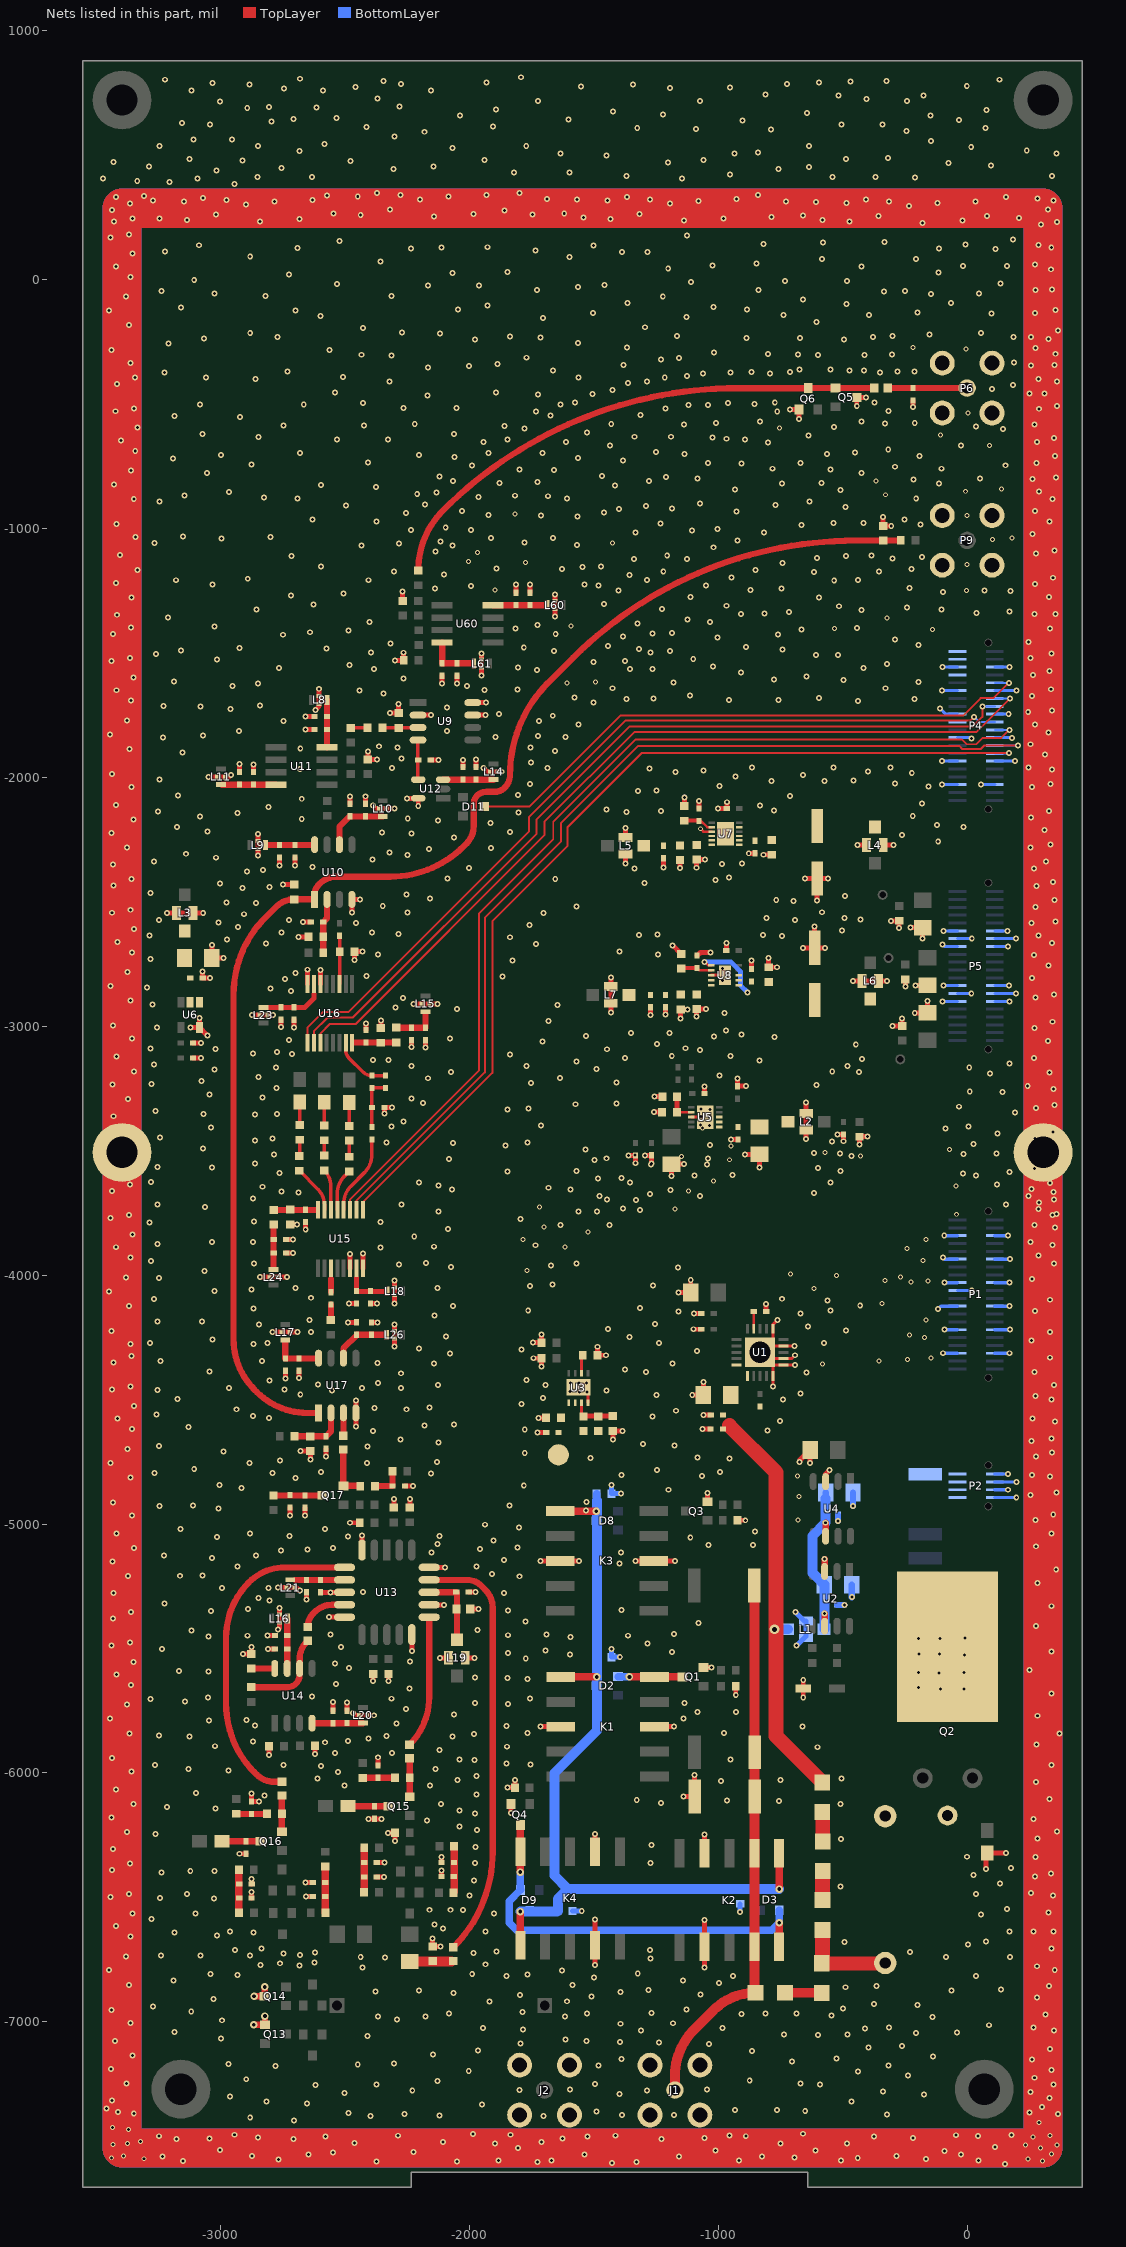
[diagram p0: the nets of this part, all layers, seen from the top]
# Altium PCB MISC109358.PcbDoc (part 5 of 7)
Units mil, origin at the board's own origin, x right, y up, seen from the top; angles counter-clockwise.
Board outline 4015.75 x 8543.31 mil, 4 copper layers (TopLayer, GND, POWER, BottomLayer), stack 33.234 mil thick; 299 components, 170 nets, 998 pads, 2318 vias.

## Via types
v1: diameter 24, hole 12, TopLayer to BottomLayer, 2184 vias
v2: diameter 20, hole 12, TopLayer to BottomLayer, 95 vias
v3: diameter 30, hole 15, TopLayer to BottomLayer, 37 vias
v4: diameter 40, hole 20, TopLayer to BottomLayer, 2 vias

## Nets (pads, with @x,y where several pads share a name; then routed paths per layer and width w, separated by ;. In a path a pad name is that pad's centre, name@x,y a point inside that pad or via, vN(x,y) a via of type N, cw(c..) or ccw(c..) an arc to the next point about the centre after c; other vN are vias at no path point) (continued)
GND: (continued)
  other v1: -2432.52,-301.52 -679,-301 -301,-301 -800,-299 355.48,-297.52 -1018,-292 -3438.52,-282.52 -2562.52,-282.52 275.48,-273.52 -1367.52,-271.52 -3208.52,-255.52 -1563.52,-254.52 -495.52,-240.52 -1977.52,-239.52 327.48,-238.52 -3066.52,-236.52 -887,-234 -671.52,-233.52 -1715,-232 -2770.52,-230.52 -379,-230 185.48,-230.52 257.48,-229.52 -1836.52,-227.52 -1165,-227 -299.52,-225.52 -150.52,-220.52 -2117.52,-216.52 -2880.52,-214.52 56.48,-214.52 -2270.52,-211.52 365.48,-204.52 -2426.85,-193.52 -1295,-191 -3368.52,-182.52 -606,-169 -1704.52,-154.52 -1127,-150 -2597.52,-145.52 -738,-142 -395,-142 97,-136 -1503,-134 272,-134 -199,-132 -3447.52,-123.52 -2699.52,-123.52 355,-122 -2045.52,-120.52 -884,-119 -3159.3,-111.52 -1020,-109 -1926.52,-103.52 -485,-97 -1365,-93 -64,-93 -660,-80 -1223,-68 -3379.52,-67.52 -2819.52,-65.52 -2313.52,-65.52 -146,-57 47,-55 -3023.52,-54.52 -335,-47 -3236.52,-45.52 -249,-45 274,-42 -839,-41 -1728.52,-40.52 341,-39 -1563,-29 -2165.52,-23.52 -1961.52,-23.52 -1458,-21 -2532.16,-17.52 134,-16 -1110,-10 -732,-6 -483,-6 -3105.52,-1.52 -3362.52,11.48 -2724.52,21.48 -2068.52,27.48 -115,29 -1847.31,30.48 337,42 -1201,45 -425,53 -3420.52,53.48 -16,56 161,56 -1024,58 273,62 -847,66 -2356.52,73.48 -584,84 -205,84 -1598,91 -2880.52,92.48 -3353.52,104.48 -1386,111 -1285,111 -3222.52,113.48 -1734.52,116.48 113,123 -2234,124.48 -113,125 -2691.52,127.48 -2111.52,129.48 338,130 -1927.52,130.48 -1501,138 -3085.52,138.48 286,140 -6,142 -818,144 -580,150 -333,152 -2522.52,155.48 185,162 -3441.52,170.48 -1125,177 -3367.52,182.48 297.48,221.48 -178.52,228.48 360.48,231.48 -3427.52,233.48 -2841.52,234.48 -472.52,234.48 -1138.52,237.48 -19.52,237.48 -3135.52,240.48 -581.52,240.48 -2682.52,243.48 -1432.52,243.48 -3354.52,245.48 -3244.52,246.48 -979.52,246.48 208.48,247.48 -1541.52,249.48 -785.52,252.48 -2142.52,254.48 -355.52,255.48 79.48,255.48 -658.83,257.48 -2436.52,260.48 -3018.52,261.48 -1745.52,261.48 -1983.52,263.48 -1315.52,264.48 -2545.52,266.48 -1618.83,266.48 -1858.52,278.48 -3435.52,279.48 -2319.52,281.48 324.48,281.48 -234.52,296.48 -2897.52,302.48 -3363.52,305.48 -1194.52,305.48 -119.52,307.48 -484.52,308.48 -607.52,312.48 -2782.52,313.48 -313.52,313.48 -3147.52,314.48 -727.52,314.48 33.48,314.48 -1079.52,316.48 -1444.52,317.48 -3270.52,318.48 346.48,318.48 -2976.52,319.48 -2629.52,320.48 -1567.52,321.48 -2198.52,322.48 -1273.52,322.48 -406.52,322.48 -1687.52,323.48 -926.52,323.48 282.03,325.48 -3069.52,328.48 -3419.52,331.48 -1366.52,331.48 155.48,332.48 -2083.52,333.48 -2448.52,334.48 -3308.19,336.48 -2571.52,338.48 -2277.52,339.48 -839.52,339.48 -1930.52,340.48 -2370.52,348.48 -1799.52,348.48 -2943.52,384.48 -3205.52,393.48 -3334.52,397.48 -3471.52,406.48 -3091.52,407.48 -1145.52,407.48 -209.52,411.48 -2851.52,413.48 -2631.52,413.48 -540.52,413.48 -367.52,413.48 -1369.52,417.48 340.48,417.48 -952.52,423.48 -1820.52,430.48 -1598.52,430.48 -3015.52,439.48 -2305.52,445.48 -757.52,445.48 -2755.52,449.48 -634.52,453.48 -3286.52,455.48 -2144.52,455.48 96.48,458.48 -74.52,468.48 -1201.52,470.48 -3429.52,473.48 -2477,477.48 -2911.52,478.48 -1939.52,481.48 -1058.52,481.48 -3124.52,485.48 -486.52,485.48 -317.52,488.48 -1448.52,498.48 -1634.52,507.48 -934.52,507.48 359.48,507.48 -839.52,511.48 -2682,517.48 239.48,518.48 -2068.52,528.48 16.48,532.48 -3244.52,537.48 -2849.52,537.48 -1771.52,537.48 -635.52,537.48 -2582.52,545.48 -144.52,556.48 -2954.52,562.48 -3108.52,563.48 -2300.52,575.48 -2179.52,594.48 -243.52,597.48 -787.52,603.48 -1088.52,605.48 -1325.52,609.48 74.48,609.48 -2413.52,613.48 -1904.52,616.48 -3041.52,624.48 -505.52,624.48 -340.52,624.48 -3154.52,629.48 -2795.52,636.48 -902.52,639.48 -33.52,641.48 -1602.52,643.48 -2706.52,646.48 -2533.52,650.48 -2038.52,660.48 -147.52,660.48 -1221.52,663.48 -642.52,669.48 -1423.52,676.48 78.48,682.48 -1893.52,684.48 -2892.52,690.48 -2614.52,691.48 -2804.52,694.48 -2281.52,695.48 -3002.52,716.48 -1724.52,718.48 -1074,718.48 -241.52,718.48 -403.98,725.48 -2369.52,728.48 -517.52,739.48 -174.52,740.48 -810.52,744.48 -3116.52,759.48 -2588.52,759.48 -2153.52,759.48 -2744.52,767.48 -1194.52,769.48 -953.52,772.48 -2458.52,774.48 -1551.52,776.48 -1.52,778.48 -2883.52,784.48 -1342.52,784.48 -2274.06,786.48 -724.52,786.48 -3032.52,789.48 -1931.52,791.48 -595.52,791.48 -468.52,795.48 -323.52,797.48 -2345.52,798.48 -3222.52,803.48 129.48,803.48 -2680.52,807.48 -1793.52,813.48
  other v2: 302,-7559 245,-7551 -3308,-7550 -3438,-7546 -3390,-7539 339,-7531 295,-7506.52 235,-7495 362,-7495 -3432,-7493 -3373,-7489 -3321,-7480 265,-7462 333,-7456 -3370,-7432 -3434,-7424 288,-7405 -679,-4983 -676,-4889 -681,-4806 -581,-4356 -354,-4344 -240,-4338 -146,-4333 -171,-4250 -232,-4241 -165,-4179 -342,-4114 -615,-4054 -225,-4028 -158,-4023 -331,-4021 -267,-4008 -524,-4002 -710,-3995 -1768,-3981 -177,-3941 -242,-3892 -1616,-3886 -1784,-3856 -166,-3856 -1523,-3827 -1700,-3806 -42,-3755 -1173,-3734 -1719,-3726 -1119,-3662 -44,-3641 -1020,-3622 -954,-3536 -1148,-3523 -428,-3521 -1334,-3517 -571,-3507 -71,-3494 -949,-3481 -1064,-3408 -1607,-1621 -1494,-1616 -139,-1406 -533,-1401 -1592,-1391 -322,-1359 -2,-1249 -1898,-1247 0,-1144 -1774,-1137 -2004,-1132 -1967,-1096 -1424,-1058 102,-1043 181,-1037 -1,-947 -1816,-941 -328,-864 -7,-850 138,-841 -366,-809 89,-666 -108,-624 -754,-596 3,-536 -4,-279 -217,-272
GPOS1: C72.1 C96.1 R56.1 U10.1 U17.1 | length 5556.2
  TopLayer w25: U10.1@-2622.48,-2489.52 C72.1@-2704.52,-2489.52 C72.1@-2704.52,-2489.52 ccw(c-2704.58,-2589.52) -2775.29,-2518.81 -2820.26,-2563.78 ccw(c-2513.03,-2871.01) -2947.52,-2871.01 -2947.52,-4256.99 ccw(c-2661.35,-4256.99) -2863.7,-4459.34 -2853.2,-4469.84 ccw(c-2652.44,-4269.08) -2652.44,-4553 U17.1@-2606,-4553 ; U10.1@-2622,-2490 -2622,-2470.15 cw(c-2567.37,-2470.15) -2606,-2431.52 -2602.29,-2427.81 cw(c-2531.58,-2498.52) -2531.58,-2398.52 -2317.24,-2398.52 ccw(c-2317.24,-1981.54) -2022.39,-2276.39 -2011.81,-2265.81 ccw(c-2082.52,-2195.1) -1982.52,-2195.1 -1982.52,-2105.52 cw(c-1936.6,-2105.52) -1969.07,-2073.05 cw(c-1931.57,-2110.55) -1931.57,-2057.52 -1897.22,-2057.52 ccw(c-1897.22,-2002.89) -1858.59,-2041.52 ccw(c-1911.88,-1988.23) -1836.52,-1988.23 cw(c-1315.75,-1988.23) -1683.99,-1619.99 -1583.25,-1519.25 cw(c-445.99,-2656.51) -445.99,-1048.18 C96.1@-337.61,-1048.18 ; C96.1@-353.41,-1048.18 C96.1@-337.61,-1048.18 ; R56.1@-266.61,-1047.18 cw(c-269.02,-1044.77) -269.02,-1048.18 C96.1@-337.61,-1048.18
H5V: C16.2 C17.2 C20.2 C21.2 C22.2 C25.1 C26.1 D2.3 D3.3 D8.3 D9.3 K1.1 K2.1 K3.1 K4.1 R11.2 TP1.1 U3.1 U3.2 | length 3356.3
  TopLayer w30: K4.1@-1795.46,-6692.12 v3(-1795.46,-6556.96) ; K3.1@-1635.12,-4948.14 v3(-1489.9,-4948.14) ; K1.1@-1632.12,-5614.14 -1631.99,-5614.01 v3(-1488.14,-5614.01) ; v3(-755.14,-6466.44) K2.1@-755.14,-6322.4
  BottomLayer w30: -1489.9,-4905.59 -1489.9,-4904.52 ; -1488.83,-4904.52 C20.2@-1488.83,-4877.52
  BottomLayer w40: v3(-1795.46,-6556.96) -1647.27,-6556.96 C21.2@-1644.83,-6554.52 -1644.83,-6506.52 -1604.52,-6466.21 ; -1487.83,-4905.59 C16.2@-1487.83,-5534.52 -1487.83,-5829.83 -1658.52,-6000.52 -1658.52,-6412.21 -1604.52,-6466.21 ; C17.2@-912.52,-6466.44 v3(-755.14,-6466.44) ; C17.2@-912.52,-6466.21 -1604.52,-6466.21
  other v1: -1530.52,-4944.52 -1529.52,-4911.52
H12V: C7.1 C8.1 C9.1 D1.2 L1.1 R1.1 U1.1 U1.20 | length 1642
  TopLayer w60: -955.52,-4604.52 -767.52,-4792.52 -767.52,-5852.08 D1.2@-582.11,-6037.49
  BottomLayer w40: v4(-774.88,-5422.52) L1.1@-720.52,-5422.52
"HP FILT EN": P4.4
HT: P2.2 P2.4 P2.6 P2.8 R3.2
IN1: P4.20
IN2: P4.8
K0: D11.3 P4.9 | length 2370.5
  TopLayer w8: D11.3@-1940.52,-2117.02 -1860.02,-2117.02 -1759.02,-2117.02 -1392.52,-1750.52 -14.52,-1750.52 54.48,-1681.52 105.48,-1681.52 v1(167.48,-1619.52)
  BottomLayer w8: P4.9@111.04,-1619.5 v1(167.48,-1619.52)
LB_A0: P4.27 U15.9 | length 4036.4
  TopLayer w8: U15.9@-2428.38,-3736.3 -2428.38,-3707.38 -1908,-3187 -1908,-2577 -1605,-2274 -1605,-2199 -1308.52,-1902.52 -1035,-1902.52 ; -1241.14,-1902.52 -1035,-1902.52 ; v1(167.48,-1902.52) -1035,-1902.52
  BottomLayer w8: P4.27@111.04,-1902.97 167.03,-1902.97 v1(167.48,-1902.52)
LB_A1: P4.25 U15.10 | length 3960.5
  TopLayer w8: U15.10@-2453.97,-3736.3 -2453.97,-3700.97 -1938,-3185 -1938,-2564 -1632,-2258 -1632,-2184 -1321,-1873 -32.04,-1873 -19.52,-1885.52 55.48,-1885.52 69.53,-1871.47 v1(203.48,-1871.47)
  BottomLayer w8: P4.25@111.04,-1871.47 v1(203.48,-1871.47)
LB_A2: P4.21 U15.11 | length 3955.9
  TopLayer w8: U15.11@-2479.56,-3736.3 -2479.56,-3695.56 -1962,-3178 -1962,-2548 -1663,-2249 -1663,-2178 -1333,-1848 -20.04,-1848 -1.52,-1866.52 37.48,-1866.52 63.48,-1840.52 137.48,-1840.52 v1(169.48,-1808.52)
  BottomLayer w8: P4.21@111.04,-1808.48 P4.21@111.04,-1808.48 v1(169.48,-1808.52)
LB_A4: P4.19 U16.9 | length 3412
  TopLayer w8: U16.9@-2650.14,-3066.22 -2650.14,-3004.14 -2587.52,-2941.52 -2485.52,-2941.52 -1760,-2216 -1760,-2158 -1373.52,-1771.52 -1251,-1771.52 ; -1280.52,-1771.52 -1251,-1771.52 ; v1(27.48,-1756.52) 12.48,-1771.52 -1251,-1771.52
  BottomLayer w8: v1(27.48,-1756.52) 47.94,-1776.98 P4.19@111.04,-1776.98
LB_A5: P4.15 U16.10 | length 3381.2
  TopLayer w8: U16.10@-2624.55,-3066.22 -2624.55,-3019.55 -2569.52,-2964.52 -2469.21,-2964.52 -1730,-2225.31 -1730,-2168 -1356.52,-1794.52 23.42,-1794.52 61.48,-1756.46 v1(61.48,-1714.52)
  BottomLayer w8: v1(61.48,-1714.52) 62.01,-1713.99 P4.15@111.04,-1713.99
LB_A6: P4.13 U16.11 | length 3507.5
  TopLayer w8: U16.11@-2598.96,-3066.22 -2598.96,-3028.96 -2560.52,-2990.52 -2457.4,-2990.52 -1698.52,-2231.63 -1698.52,-2178.52 -1337.52,-1817.52 -1207,-1817.52 ; -1255.52,-1817.52 -1207,-1817.52 ; v1(172.48,-1682.52) 37.48,-1817.52 -1207,-1817.52
  BottomLayer w8: P4.13@111.04,-1682.5 v1(172.48,-1682.52)
LB_IN1: R72.1 U15.13 | length 168.3
  TopLayer w14: U15.13@-2530.74,-3736.3 -2530.74,-3671.99 cw(c-2430.74,-3671.99) -2501.45,-3601.28 R72.1@-2483.48,-3583.31
LB_IN2: R77.2 U15.14 | length 164.7
  TopLayer w14: R77.2@-2583.52,-3578.83 cw(c-2649.16,-3644.47) -2556.33,-3644.47 U15.14@-2556.33,-3736.3
LB_IN3: R79.2 U15.15 | length 194.5
  TopLayer w14: R79.2@-2683.48,-3580.31 cw(c-2683.48,-3582.12) -2682.2,-3580.84 -2608.52,-3654.52 cw(c-2672.74,-3718.74) -2581.92,-3718.74 U15.15@-2581.92,-3736.3
LB_IN4: R68.1 U15.12 | length 320
  TopLayer w14: U15.12@-2505.15,-3736.3 -2505.15,-3712.57 cw(c-2405.15,-3712.57) -2475.86,-3641.86 -2421.29,-3587.29 ccw(c-2492,-3516.58) -2392,-3516.58 R68.1@-2392,-3454.52
LB_OUT: R33.1 R41.2 U16.3 | length 193.8
  TopLayer w14: U16.3@-2521.52,-2829.33 R33.1@-2521.52,-2635.52
"LP FILT EN": P4.2
NetC6_1: C6.1 U1.14 | length 68.5
  TopLayer w12: U1.14@-857.41,-4215.02 C6.1@-857.41,-4146.52
NetC14_1: C14.1 C15.1 C28.1 C29.1 L1.3 U2.6 U4.6 | length 696
  TopLayer w25: U2.6@-572.51,-5410.24 v1(-572.51,-5359.53) ; U4.6@-568.51,-5048.65 v1(-568.51,-4994.53)
  BottomLayer w25: C15.1@-568.52,-4896.52 C15.1@-568.52,-4872.52
  BottomLayer w40: L1.3@-573.52,-5421.85 C29.1@-573.52,-5243.52 -621.52,-5195.52 -621.52,-5047.54 v1(-568.51,-4994.53) C15.1@-568.51,-4896.53
NetC18_1: C18.1 Q2.2 Q2.4 R4.2
  other v1: -108,-5663 -13,-5662 -195,-5657 -112.52,-5597.52 -194.52,-5595.52 -12.52,-5595.52 -11.52,-5525.52 -193.52,-5522.52 -111.52,-5522.52 -109.52,-5460.52 -195,-5459 -9,-5458
NetC18_2: C18.2 D5.2 D6.2 | length 381.8
  TopLayer w60: D5.2@-581.11,-6635.73 -581.11,-6766.49 C18.2@-330.05,-6764.49
NetC22_1: C22.1 R11.1 R15.1 U3.3 | length 164.2
  TopLayer w11: R11.1@-1549.3,-4559.14 U3.3@-1549.3,-4511.96
  TopLayer w20: R11.1@-1540.48,-4565.96 R15.1@-1423.48,-4565.96
NetC27_1: C27.1 U3.6 | length 67.5
  TopLayer w11: U3.6@-1549.3,-4393.81 C27.1@-1549.3,-4326.3
NetC31_1: C31.1 R20.1 U5.7 | length 117.5
  TopLayer w11: R20.1@-1164.17,-3344.94 U5.7@-1107.68,-3344.94
  TopLayer w20: R20.1@-1165.38,-3343.73 C31.1@-1165.38,-3282.73
NetC32_1: C32.1 C33.1 L2.1 U5.1 U5.2 U5.3
NetC39_1: C39.1 C40.2 L3.3 U6.1 U6.2
NetC45_2: C45.2 C46.1 C49.2 L4.3 U7.1 U7.2 U7.3 U7.5 U7.13
NetC47_1: C47.1 C48.2 C334.2 L5.1 U7.10 U7.11 U7.12
NetC53_1: C53.1 R23.1 U7.8 | length 120
  TopLayer w10: R23.1@-1077,-2174.59 -1069.45,-2174.59 -1044.33,-2199.71 U7.8@-1026.16,-2199.71
  TopLayer w16: C53.1@-1138.27,-2173.27 R23.1@-1079.51,-2173.27
NetC56_1: C56.1 C57.2 P6.5 | length 318
  TopLayer w25: C56.1@-318.04,-435.37 C57.2@-217,-435.37 P6.5@0,-435.37
NetC56_2: C56.2 Q5.1 Q6.3 R26.2 | length 2130.4
  TopLayer w25: R26.2@-2205.52,-1168.21 cw(c-1863.45,-1168.21) -2105.33,-926.33 cw(c-921.3,-2110.36) -921.3,-435.89 Q6.3@-638.02,-435.89 ; Q6.3@-637.02,-434.89 C56.2@-373.64,-434.89
NetC58_1: C58.1 C61.2 C63.1 C64.2 L7.1 U8.9 U8.10
NetC59_2: C59.2 C60.1 C62.1 L6.3 U8.1 U8.2 U8.3 U8.6 | length 287.5
  TopLayer w10: v1(-1054.52,-2740.52) -1039.78,-2755.26 U8.6@-1028.89,-2755.26
  BottomLayer w20: v1(-1054.52,-2740.52) -949.52,-2740.52 -911.1,-2778.93 -911.1,-2834.93 v1(-882.52,-2863.52)
NetC65_2: C65.2 R25.1 U8.7 | length 122.4
  TopLayer w10: R25.1@-1084.58,-2765.83 -1075.47,-2774.94 U8.7@-1028.89,-2774.94
  TopLayer w16: C65.2@-1147.52,-2765.83 R25.1@-1084.58,-2765.83
NetC66_2: C66.2 C67.1 L8.1 U11.8 | length 190.5
  TopLayer w25: U11.8@-2572,-1879 C67.1@-2572,-1808 C66.2@-2572,-1754.08 L8.1@-2572,-1688.52
NetC68_2: C68.2 C69.1 L9.3 U10.8 | length 191
  TopLayer w25: L9.3@-2814.52,-2271.52 U10.8@-2623.52,-2271.52
NetC70_1: C70.1 R39.1 U9.3 | length 143.3
  TopLayer w14: C70.1@-2349.52,-1800.52 cw(c-2347.11,-1802.93) -2347.11,-1799.52 U9.3@-2206.52,-1799.52
NetC70_2: C70.2 R29.1 | length 68.2
  TopLayer w14: R29.1@-2477,-1800.52 C70.2@-2408.83,-1800.52
NetC71_1: C71.1 U13.17 | length 1725.2
  TopLayer w25: U13.17@-2161.46,-5224.12 -2009.02,-5224.12 cw(c-2009.02,-5304.02) -1952.52,-5247.52 -1935.81,-5264.23 cw(c-2006.52,-5334.94) -1906.52,-5334.94 -1906.52,-6319.07 cw(c-2445.97,-6319.07) C71.1@-2064.52,-6700.52
NetC71_2: C71.2 R37.1 R42.2 | length 168.1
  TopLayer w40: R37.1@-2239.52,-6757.52 C71.2@-2071.4,-6757.52
NetC73_1: C73.1 R28.2 R40.2 U10.2 | length 219.6
  TopLayer w25: C73.1@-2587.52,-2581.52 -2572,-2566 U10.2@-2572,-2490 ; R28.2@-2587.21,-2703.52 R40.2@-2587.21,-2640.52 C73.1@-2587.21,-2581.83
NetC74_1: C74.1 C75.2 L10.3 U10.6 | length 263.3
  TopLayer w25: U10.6@-2522,-2270 -2522,-2197.7 -2480.81,-2156.51 L10.3@-2348.08,-2156.51
NetC76_1: C76.1 C77.2 L11.1 U11.4 | length 216.5
  TopLayer w25: L11.1@-2993.52,-2029 U11.4@-2777,-2029
NetC78_2: C78.2 C79.2 R43.1 R47.2 | length 178.7
  TopLayer w30: R47.2@-2422.52,-6478.21 C79.2@-2422.52,-6417.52 C78.2@-2422.52,-6360.52 R43.1@-2422.52,-6299.52
NetC80_1: C80.1 C81.2 R44.2 R48.1 | length 184.7
  TopLayer w30: R48.1@-2061.21,-6478.21 R44.2@-2061.21,-6293.52
NetC82_2: C82.2 C83.1 R45.2 R49.1 | length 172.1
  TopLayer w30: R49.1@-2925.83,-6561.58 R45.2@-2925.83,-6389.52
NetC84_2: C84.2 C85.2 R46.2 R50.2 | length 180
  TopLayer w30: R50.2@-2578.21,-6562 R46.2@-2578.21,-6382
NetC86_1: C86.1 U9.4 U12.4 | length 158.2
  TopLayer w14: U12.4@-2206.52,-2007.74 U9.4@-2206.52,-1849.52
NetC87_1: C87.1 U13.14 | length 532.8
  TopLayer w25: C87.1@-2240.02,-5885.88 ccw(c-2429.68,-5696.22) -2161.46,-5696.22 U13.14@-2161.46,-5374.12
NetC87_2: C87.2 Q15.2 R52.1 | length 151.9
  TopLayer w25: Q15.2@-2239.52,-6096 C87.2@-2239.52,-5944.12
NetC88_1: C88.1 U13.4 | length 1336.2
  TopLayer w25: -2866.66,-5994.34 cw(c-2588.72,-5722.47) -2977.52,-5722.47 -2977.52,-5455.39 cw(c-2663.98,-5455.39) -2885.69,-5233.69 cw(c-2741.87,-5377.5) -2741.87,-5174.12 U13.4@-2501.46,-5174.12 ; -2863.64,-5997.4 -2854.81,-6006.23 ccw(c-2784.1,-5935.52) -2784.1,-6035.52 C88.1@-2753.52,-6035.52
NetC88_2: C88.2 Q16.2 R53.2 | length 145.8
  TopLayer w25: Q16.2@-2753.52,-6236.48 C88.2@-2753.52,-6090.64
NetC89_2: C89.2 C90.1 L14.3 U12.3 | length 202.6
  TopLayer w25: U12.3@-2105.42,-2008.84 L14.3@-1902.85,-2008.84
NetC91_1: C91.1 L12.2 Q15.3 | length 152.3
  TopLayer w25: L12.2@-2476.52,-6134.52 cw(c-2474.06,-6136.98) -2474.06,-6133.5 Q15.3@-2324.52,-6133.5
NetC92_1: C92.1 L13.2 Q16.3 | length 155.1
  TopLayer w25: L13.2@-2993.52,-6274.52 cw(c-2992.22,-6275.82) -2992.22,-6273.98 Q16.3@-2838.52,-6273.98
NetC93_2: C93.2 R52.2 R54.1 | length 129.9
  TopLayer w25: R54.1@-2428.52,-6019.48 C93.2@-2368.04,-6019.48 -2301.15,-6019.48 ccw(c-2301.15,-6016.2) R52.2@-2298.83,-6018.52
NetC94_2: C94.2 R53.1 R55.2 | length 124.2
  TopLayer w20: R55.2@-2936.52,-6163.79 ccw(c-2934.85,-6162.12) R55.2@-2934.85,-6164.48
  TopLayer w25: R55.2@-2934.85,-6164.48 C94.2@-2874.52,-6164.48 R53.1@-2812.52,-6164.48
NetC95_1: C95.1 R59.2 U14.6 | length 369
  TopLayer w25: R59.2@-2876.52,-5655.21 -2730.57,-5655.21 ccw(c-2730.57,-5608.47) -2697.52,-5641.52 ccw(c-2734.99,-5604.05) -2682,-5604.05 U14.6@-2682,-5580 -2682,-5542.42 cw(c-2582,-5542.42) -2652.71,-5471.71 C95.1@-2649.52,-5468.52
NetC95_2: C95.2 U13.7 | length 196.3
  TopLayer w25: C95.2@-2649.52,-5413.4 cw(c-2571.31,-5413.4) -2626.61,-5358.1 -2621.92,-5353.4 cw(c-2551.21,-5424.12) -2551.21,-5324.12 U13.7@-2501.46,-5324.12
NetC97_2: C97.2 R57.2 R58.2 | length 130.2
  TopLayer w25: R57.2@-2379.21,-4847.52 -2378.9,-4847.21 -2308.83,-4847.21 R58.2@-2308.83,-4787.52
NetC98_1: C98.1 C106.1 U16.15 | length 238.3
  TopLayer w14: U16.15@-2496.6,-3066.22 -2496.6,-3095.85 ccw(c-2451.81,-3095.85) -2483.48,-3127.52 -2428.58,-3182.42 ccw(c-2390.96,-3144.79) C98.1@-2390.96,-3198 cw(c-2389.8,-3199.16) -2389.8,-3197.52 C106.1@-2337,-3197.52
NetC98_2: C98.2 C103.2 C106.2 R68.2 | length 210.4
  TopLayer w14: R68.2@-2392,-3404.52 ccw(c-2393.16,-3403.36) -2391.52,-3403.36 C103.2@-2391.52,-3325.52 -2391.52,-3251.67 cw(c-2385.65,-3251.67) -2389.8,-3247.52 C106.2@-2337,-3247.52
NetC99_2: C99.2 C102.2 L17.3 U17.8 | length 199.5
  TopLayer w25: C99.2@-2739.52,-4334.53 U17.8@-2607.53,-4334.53 ; C99.2@-2739.52,-4334.04 L17.3@-2739.52,-4266.52
NetC100_2: C100.2 C101.1 L15.3 R62.2 | length 173.5
  TopLayer w25: R62.2@-2293.52,-3005.21 -2176.83,-3005.21 -2176.52,-3004.9 L15.3@-2176.52,-2948.52
NetC104_2: C104.2 C105.2 L16.3 U14.7 | length 200
  TopLayer w25: U14.7@-2732,-5580 C105.2@-2732,-5502 L16.3@-2732,-5379.99
NetC107_1: C107.1 U15.3 | length 52.2
  TopLayer w25: C107.1@-2556.33,-4067.67 -2556.33,-4015.52
NetC107_2: C107.2 R70.2 | length 60.7
  TopLayer w25: R70.2@-2556,-4178.69 C107.2@-2556,-4118
NetC108_2: C108.2 C112.2 L20.1 U14.4 | length 203.3
  TopLayer w25: U14.4@-2632,-5800 C108.2@-2547.04,-5800 L20.1@-2428.68,-5800
NetC109_1: C109.1 Q17.2 R57.1 | length 214.1
  TopLayer w25: C109.1@-2506.52,-4700.52 -2506.52,-4845.96 -2440.08,-4845.96 R57.1@-2438.52,-4847.52
NetC109_2: C109.2 U17.3 | length 91.9
  TopLayer w25: C109.2@-2506,-4644.88 U17.3@-2506,-4553
NetC110_2: C110.2 U14.8 | length 93.6
  TopLayer w25: C110.2@-2875.52,-5580.48 -2783.15,-5580.48 ccw(c-2783.15,-5578.85) U14.8@-2782,-5580
NetC111_1: C111.1 L22.1 | length 94
  TopLayer w14: C111.1@-2483.48,-3400 L22.1@-2483.48,-3306
NetC111_2: C111.2 R72.2 | length 64.7
  TopLayer w14: R72.2@-2483.48,-3524 C111.2@-2483.48,-3459.31
NetC113_1: C113.1 C114.2 L19.1 U13.16 | length 299.9
  TopLayer w25: U13.16@-2161.46,-5274.12 C114.2@-2053.12,-5274.12 ; C114.2@-2053.12,-5276 -2050.04,-5276 L19.1@-2050.04,-5464.52
NetC115_1: C115.1 R67.1 R75.2 U17.2 | length 229.6
  TopLayer w25: R67.1@-2702.52,-4646.52 -2701.83,-4647.21 R75.2@-2638.52,-4647.21 C115.1@-2575.52,-4647.21 -2556,-4627.69 U17.2@-2556,-4553
NetC116_2: C116.2 C117.2 Q17.3 R73.1 | length 196.5
  TopLayer w25: R73.1@-2787,-4884.5 Q17.3@-2590.48,-4884.5
NetC118_2: C118.2 C120.2 L21.3 U13.5 | length 198
  TopLayer w25: -2699.42,-5224.12 C118.2@-2653.52,-5224.12 U13.5@-2501.46,-5224.12
NetC119_1: C119.1 L25.1 | length 93.5
  TopLayer w14: C119.1@-2582.48,-3398.48 L25.1@-2582.48,-3305
NetC119_2: C119.2 R77.1 | length 61.7
  TopLayer w14: R77.1@-2582.52,-3519.52 C119.2@-2582.52,-3457.83
NetC121_2: C121.2 C122.2 L26.3 U17.6 | length 235.3
  TopLayer w20: -2342.52,-4239 L26.3@-2332.51,-4239
  TopLayer w25: U17.6@-2506,-4333 -2506,-4294 -2451,-4239 -2342.52,-4239
NetC123_2: C123.2 C124.1 L23.3 U16.7 | length 235.7
  TopLayer w20: L23.3@-2827.52,-2923.53 -2660.53,-2923.53 -2624.55,-2887.55 -2624.55,-2869.73
NetC125_1: C125.1 L27.1 | length 92.6
  TopLayer w14: C125.1@-2682.48,-3396.31 -2682.48,-3306.41 cw(c-2679.07,-3306.41) L27.1@-2681.48,-3304
NetC125_2: C125.2 R79.1 | length 65.4
  TopLayer w14: R79.1@-2682.48,-3521 C125.2@-2682.48,-3455.62
NetC126_2: C126.2 C129.2 L24.1 R76.2 | length 174.2
  TopLayer w25: L24.1@-2786.52,-3971.04 R76.2@-2786.52,-3796.83
NetC127_2: C127.2 C128.2 L18.1 U15.7 | length 173.5
  TopLayer w20: C128.2@-2453.97,-4063.07 -2453.97,-4010.52 ; C128.2@-2452.52,-4064.52 L18.1@-2331.52,-4064.52
NetC301_1: C301.1 R62.1 R63.2 U16.16 | length 168
  TopLayer w25: -2461.52,-3064.52 R62.1@-2293.52,-3064.52
NetC302_2: C302.2 R76.1 R78.1 U15.16 | length 171
  TopLayer w25: R76.1@-2786.52,-3737.52 U15.16@-2615.52,-3737.52
NetC304_1: C304.1 C305.2 L61.1 U60.4 | length 198.2
  TopLayer w25: C304.1@-2109.19,-1541.04 C305.2@-2050.52,-1541.04 ; C304.1@-2109.23,-1540.99 U60.4@-2109.23,-1459.08 ; C305.2@-2050.52,-1540.99 -1992.99,-1540.99
NetC306_1: C306.1 C307.2 L60.1 U60.8 | length 207.3
  TopLayer w25: U60.8@-1905.31,-1308 -1698.04,-1308
NetD1_1: D1.1 D4.2 | length 115.5
  TopLayer w60: D4.2@-580.11,-6274.49 D1.1@-580.11,-6158.98
NetD2_1: D2.1 K1.10 Q1.3 | length 258.6
  TopLayer w30: v3(-1357.02,-5613.89) -1356.89,-5614.02 Q1.3@-1143.52,-5614.02
  BottomLayer w30: D2.1@-1402.02,-5613.89 v3(-1357.02,-5613.89)
NetD3_1: D3.1 D9.1 K2.10 K4.10 Q4.3 | length 1666
  TopLayer w30: v3(-1795.46,-6398.08) K4.10@-1795.46,-6316.12 Q4.3@-1795.46,-6209.96 ; K2.10@-755.14,-6698.4 v3(-755.14,-6601.9)
  BottomLayer w30: D9.1@-1795.46,-6468.58 v3(-1795.46,-6398.08) ; D9.1@-1794.52,-6469.52 -1840.52,-6515.52 -1840.52,-6601.52 -1810.52,-6631.52 -784.77,-6631.52 v3(-755.14,-6601.9) D3.1@-755.14,-6552.14
NetD4_1: D4.1 D5.1 | length 117.4
  TopLayer w60: D5.1@-580.93,-6511.06 -580.93,-6394.8 D4.1@-580.11,-6393.98
NetD6_1: D6.1 D7.2 | length 146.3
  TopLayer w40: D7.2@-731.49,-6882.93 D6.1@-585.16,-6882.93
NetD7_1: D7.1 J1.5 K2.2 K2.9 R2.1 R6.2 R14.2 | length 2193
  TopLayer w40: J1.5@-1174,-7274 -1174,-7217.63 cw(c-909.21,-7217.63) -1096.44,-7030.39 -1018.28,-6952.22 cw(c-850.98,-7119.52) D7.1@-850.98,-6882.93 ; D7.1@-855.08,-6878.83 R14.2@-855.08,-5246.52